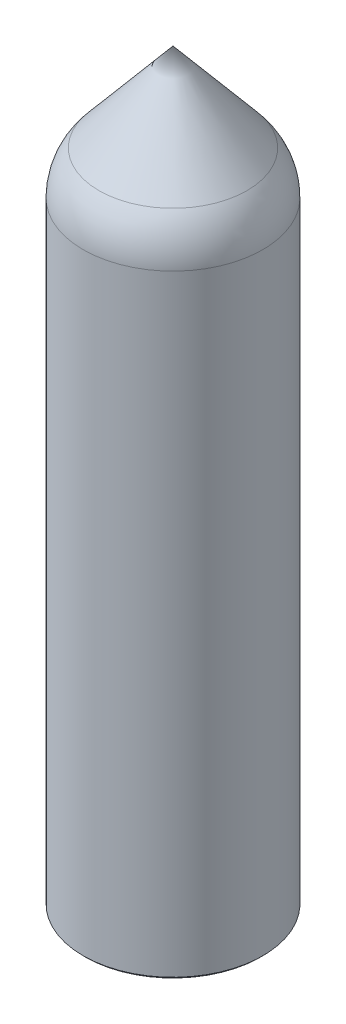
from build123d import *

# Parameters (mm, degrees)
FILLET1_R     = 15
CHAMFER1_SIZE = 0.5


with BuildPart() as part:
    # Sketch1 → Revolve1 (revolve)
    with BuildSketch(Plane.XY, mode=Mode.PRIVATE) as revolve1_sk:
        Polygon((0, 0), (-20, -23.835071852), (-20, -166), (0, -166), align=None)
    revolve(revolve1_sk.sketch.rotate(Axis((0, -166, 0), (0, 1, 0)), 270), axis=Axis((0, -166, 0), (0, 1, 0)))

    # Fillet1
    fillet1_edges = [part.edges().sort_by_distance(p)[0] for p in [
        (0, -23.835071852, 20),
    ]]
    fillet(fillet1_edges, radius=FILLET1_R)

    # Chamfer1
    chamfer1_edges = [part.edges().sort_by_distance(p)[0] for p in [
        (0, -166, 20),
    ]]
    chamfer(chamfer1_edges, length=CHAMFER1_SIZE)


solid = part.part
